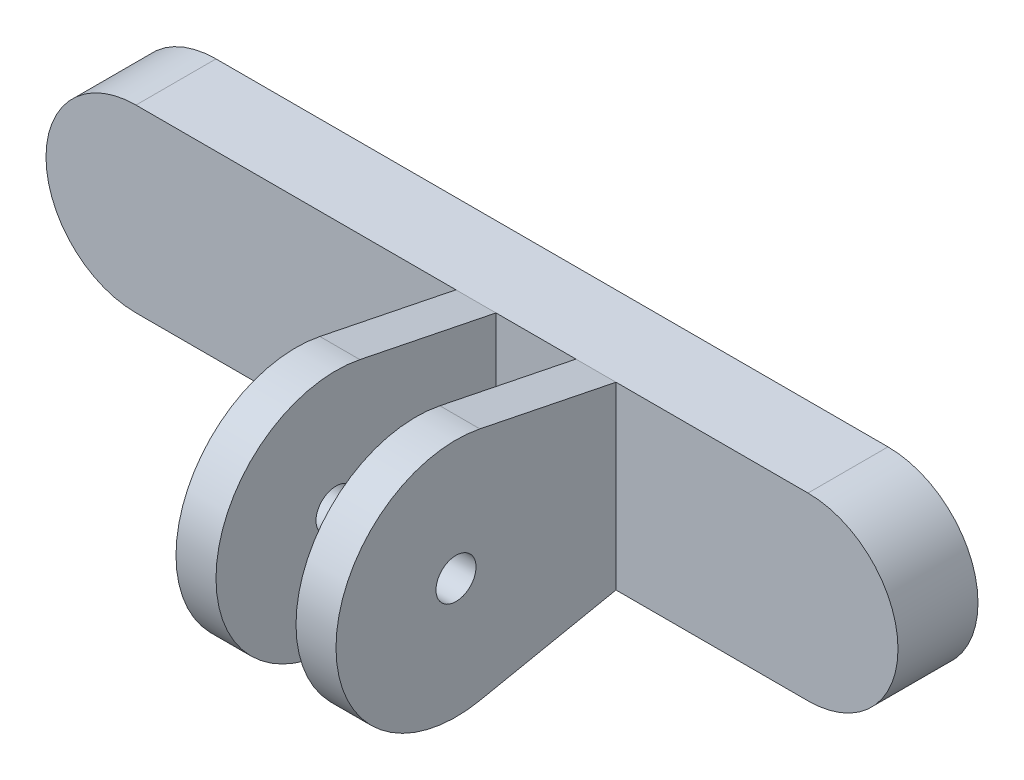
SolidWorks part; units mm, degrees
ref_plane "Front plane" through (0, 0, 0) normal (0, 0, 1) x (1, 0, 0)
ref_plane "Top plane" through (0, 0, 0) normal (0, 1, 0) x (1, 0, 0)
ref_plane "Right plane" through (0, 0, 0) normal (1, 0, 0) x (0, 0, -1)
sketch "Sketch 1" plane through (0, 0, 0) normal (0, 0, 1) x (1, 0, 0)
  line L0 (0, 0) -> (16.8, 0) construction
  line L1 (0, 2.25) -> (16.8, 2.25)
  line L2 (0, -2.25) -> (16.8, -2.25)
  arc A0 (0, 2.25) -> (0, -2.25) centre (0, 0) ccw
  arc A1 (16.8, -2.25) -> (16.8, 2.25) centre (16.8, 0) ccw
  point P3 (8.4, 0)
  point P8 (19.05, 0)
  dimension "D1" = 10.65
  dimension "D2" = 2.25
extrude "Boss-Extrude 1" add sketch "Sketch 1" along normal blind 2
sketch "Sketch 2" plane through (0, 0, 2) normal (0, 0, 1) x (1, 0, 0)
  line L0 (16.8, 2.25) -> (12, 2.25)
  line L1 (16.8, 2.25) -> (0, 2.25) construction
  dimension "D1" = 4.8
ref_plane "Reference plane 1" through (12, 0, 0) normal (-1, 0, 0) x (0, 0, 1)
sketch "Sketch 3" plane through (12, 0, 0) normal (-1, 0, 0) x (0, 0, 1)
  line L0 (2, 2.25) -> (2, -2.249)
  line L1 (2, 0.001) -> (4.2982, 0.001) construction
  line L2 (2, -2.249) -> (5.4038, -2.9392)
  line L3 (2, 2.25) -> (5.403, 2.941)
  circle A0 centre (6, 0.001) radius 0.5
  arc A1 (5.4038, -2.9392) -> (5.403, 2.941) centre (6, 0.001) ccw
  point P9 (2, 0.0005)
  dimension "D2" = 1
  dimension "D3" = 6
  dimension "D1" = 2.25
  dimension "D4" = 4
extrude "Boss-Extrude 2" add sketch "Sketch 3" along normal blind 4
sketch "Sketch 4" plane through (0, 0, 0) normal (0, 1, 0) x (1, 0, 0)
  line L0 (12, -2) -> (11, -2) construction
  line L1 (11, -2) -> (9, -2)
  line L2 (9, -2) -> (9, -10.0932)
  line L3 (9, -10.0932) -> (11, -10.0932)
  line L12 (11, -10.0932) -> (11, -2)
  dimension "D2" = 1
  dimension "D3" = 2
extrude "Cut-Extrude 1" cut sketch "Sketch 4" against normal through all both and the other way through all
